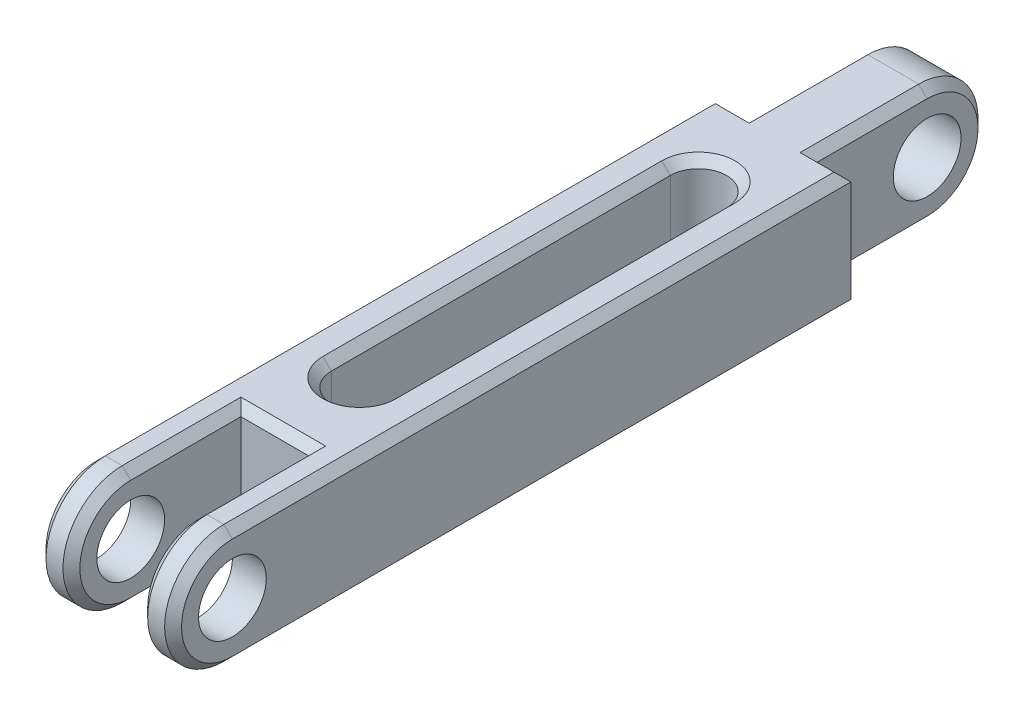
from build123d import *

# Parameters (mm, degrees)
BOSS_EXTRUDE1_DEPTH = 14
SKETCH2_R           = 4
CUT_EXTRUDE1_DEPTH  = 14
SKETCH3_R           = 4
CUT_EXTRUDE2_DEPTH  = 30
CUT_EXTRUDE3_DEPTH  = 14
CHAMFER1_SIZE       = 1
SCALE1_SCALE        = 0.5


with BuildPart() as part:
    # Sketch1 → Boss-Extrude1 (new body)
    with BuildSketch(Plane(origin=(0, 0, 0), x_dir=(1, 0, 0), z_dir=(0, 1, 0))):
        Polygon((4, 40), (8, 40), (8, -40), (4, -40), (4, -20), (-4, -20), (-4, -40), (-8, -40), (-8, 40), (-4, 40), (-4, 60), (4, 60), align=None)
    extrude(amount=BOSS_EXTRUDE1_DEPTH)

    # Sketch2 → Cut-Extrude1 (cut)
    with BuildSketch(Plane(origin=(4, 0, 0), x_dir=(0, 0, -1), z_dir=(1, 0, 0))):
        with BuildLine():
            Line((60, 14), (53, 14))
            ThreePointArc((53, 14), (57.949747468, 11.949747468), (60, 7))
            Line((60, 7), (60, 14))
        make_face()
        with BuildLine():
            Line((60, 0), (60, 7))
            ThreePointArc((60, 7), (57.949747468, 2.050252532), (53, 0))
            Line((53, 0), (60, 0))
        make_face()
        with Locations((53, 7)):
            Circle(SKETCH2_R)
    extrude(amount=-CUT_EXTRUDE1_DEPTH, mode=Mode.SUBTRACT)

    # Sketch3 → Cut-Extrude2 (cut)
    with BuildSketch(Plane(origin=(8, 0, 0), x_dir=(0, 0, -1), z_dir=(1, 0, 0))):
        with BuildLine():
            ThreePointArc((-40, 7), (-37.949747468, 11.949747468), (-33, 14))
            Line((-33, 14), (-40, 14))
            Line((-40, 14), (-40, 7))
        make_face()
        with BuildLine():
            ThreePointArc((-33, 0), (-37.949747468, 2.050252532), (-40, 7))
            Line((-40, 7), (-40, 0))
            Line((-40, 0), (-33, 0))
        make_face()
        with Locations((-33, 7)):
            Circle(SKETCH3_R)
    extrude(amount=-CUT_EXTRUDE2_DEPTH, mode=Mode.SUBTRACT)

    # Sketch4 → Cut-Extrude3 (cut)
    with BuildSketch(Plane(origin=(0, 14, 0), x_dir=(1, 0, 0), z_dir=(0, 1, 0))):
        with BuildLine():
            Line((3.320010274, 30), (3.320010274, -10))
            ThreePointArc((3.320010274, -10), (0, -13.320010274), (-3.320010274, -10))
            Line((-3.320010274, -10), (-3.320010274, 30))
            ThreePointArc((-3.320010274, 30), (0, 33.320010274), (3.320010274, 30))
        make_face()
    extrude(amount=-CUT_EXTRUDE3_DEPTH, mode=Mode.SUBTRACT)

    # Chamfer1
    chamfer1_edges = [part.edges().sort_by_distance(p)[0] for p in [
        (6, 14, -40),
        (4, 0, 26.5),
        (-8, 0, -3.5),
        (4, 14, -46.5),
        (4, 0, -46.5),
        (0, 14, -33.320010274),
        (-3.320010274, 14, -10),
        (0, 14, 13.320010274),
        (3.320010274, 14, -10),
        (-6, 14, -40),
        (-8, 14, -3.5),
        (0, 14, 20),
        (-4, 14, -46.5),
        (4, 14, 26.5),
        (4, 7, -60),
        (-4, 7, -60),
        (-4, 0, -46.5),
        (4, 7, 40),
        (-4, 14, 26.5),
        (8, 14, -3.5),
        (-8, 7, 40),
        (8, 7, 40),
        (-4, 7, 40),
        (8, 0, -3.5),
        (-4, 0, 26.5),
    ]]
    chamfer(chamfer1_edges, length=CHAMFER1_SIZE)


with BuildPart() as part_1:
    # Scale1: scaled about (0, 0, 0)
    add(part.part.scale(SCALE1_SCALE))


solid = part_1.part
